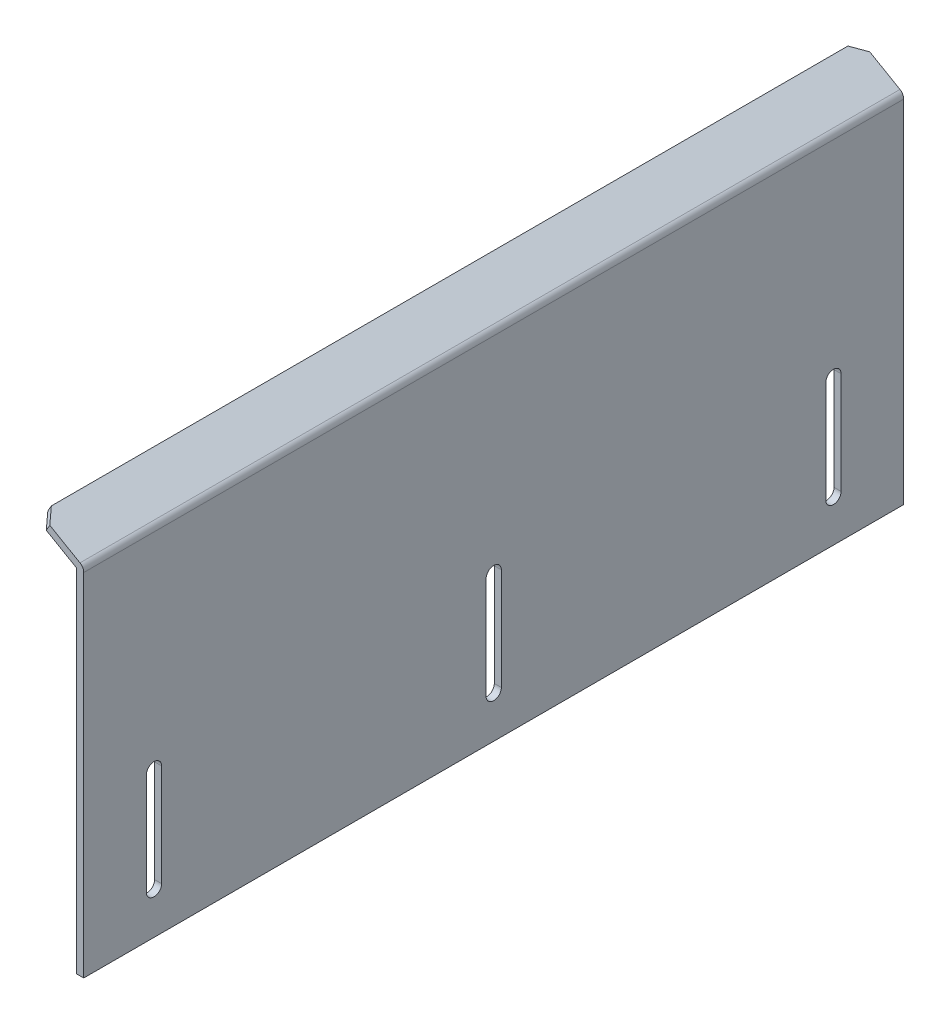
SolidWorks part; units mm, degrees
material "1023 碳钢板 (SS)"
ref_plane "前视基准面" through (0, 0, 0) normal (0, 0, 1) x (1, 0, 0)
ref_plane "上视基准面" through (0, 0, 0) normal (0, 1, 0) x (1, 0, 0)
ref_plane "右视基准面" through (0, 0, 0) normal (1, 0, 0) x (0, 0, -1)
ref_plane "基准面4" through (0, 0, 350) normal (0, 0, 1) x (1, 0, 0)
sketch "草图1" plane through (0, 0, 350) normal (0, 0, 1) x (1, 0, 0)
  line L0 (3, -150) -> (3, 1.7321)
  line L1 (3, 1.7321) -> (-15.8205, 12.5981)
  line L2 (-15.8205, 12.5981) -> (-17.3205, 10)
  line L3 (-17.3205, 10) -> (0, 0)
  line L4 (0, 0) -> (0, -150)
  line L5 (0, -150) -> (3, -150)
extrude "凸台-拉伸1" add sketch "草图1" against normal blind 350
sketch "草图2" plane through (0, 0, 0) normal (-1, 0, 0) x (0, 0, 1)
  line L0 (316.75, -88.25) -> (316.75, -131.75)
  line L1 (323.25, -131.75) -> (323.25, -88.25)
  arc A0 (316.75, -131.75) -> (323.25, -131.75) centre (320, -131.75) ccw
  arc A1 (323.25, -88.25) -> (316.75, -88.25) centre (320, -88.25) ccw
  dimension "D1" = 43.5
extrude "切除-拉伸1" cut sketch "草图2" against normal through all
sketch "草图3" plane through (0, 0, 0) normal (-1, 0, 0) x (0, 0, 1)
  line L0 (26.75, -88.25) -> (26.75, -131.75)
  line L1 (33.25, -131.75) -> (33.25, -88.25)
  arc A0 (26.75, -131.75) -> (33.25, -131.75) centre (30, -131.75) ccw
  arc A1 (33.25, -88.25) -> (26.75, -88.25) centre (30, -88.25) ccw
  dimension "D1" = 43.5
extrude "切除-拉伸2" cut sketch "草图3" against normal through all
sketch "草图4" plane through (3, 0, 0) normal (1, 0, 0) x (0, 0, -1)
  line L0 (-171.75, -131.75) -> (-171.75, -88.25)
  line L1 (-178.25, -88.25) -> (-178.25, -131.75)
  arc A0 (-178.25, -131.75) -> (-171.75, -131.75) centre (-175, -131.75) ccw
  arc A1 (-171.75, -88.25) -> (-178.25, -88.25) centre (-175, -88.25) ccw
  dimension "D1" = 43.5
extrude "切除-拉伸3" cut sketch "草图4" against normal through all
chamfer "倒角1" distance 5 angle 45 2 edges at (-16.5705, 11.299, 0) (-16.5705, 11.299, 350)
fillet "圆角1" radius 0.2 1 edges at (0, 0, 175)
fillet "圆角2" radius 3.2 1 edges at (3, 1.7321, 175)
